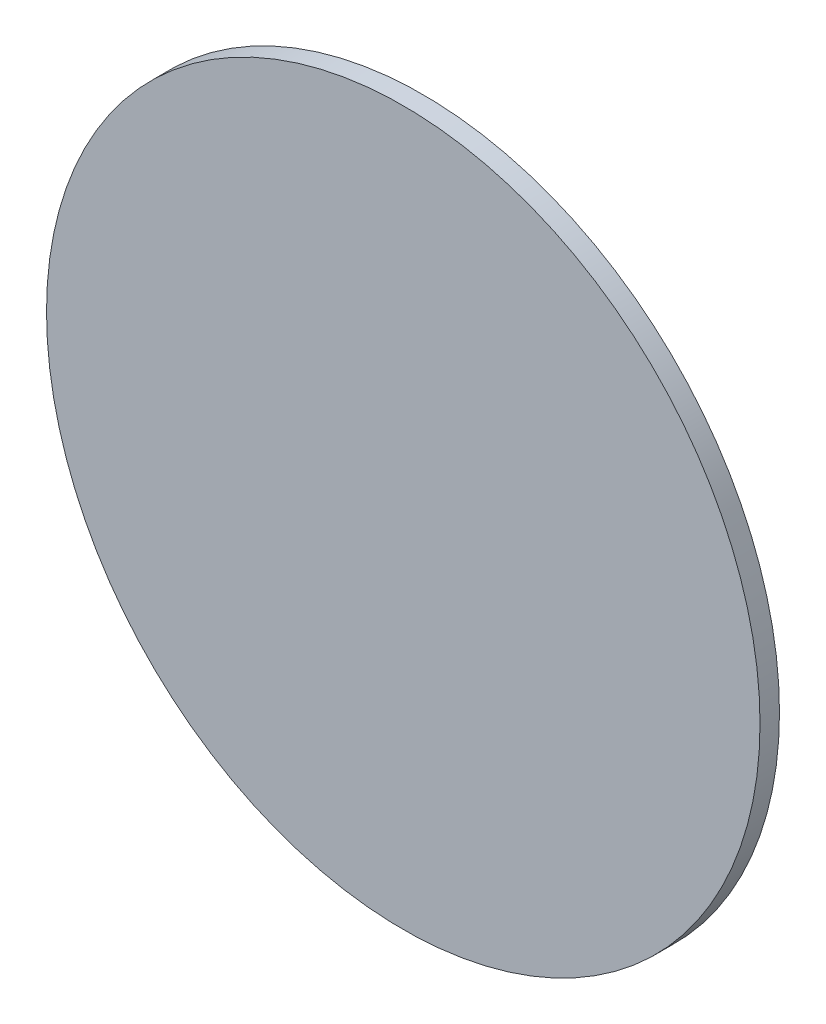
from build123d import *

# Parameters (mm, degrees)
SKETCH1_R           = 110
BOSS_EXTRUDE1_DEPTH = 6


with BuildPart() as part:
    # Sketch1 → Boss-Extrude1 (new body)
    with BuildSketch(Plane.XY):
        Circle(SKETCH1_R)
    extrude(amount=BOSS_EXTRUDE1_DEPTH)


solid = part.part
